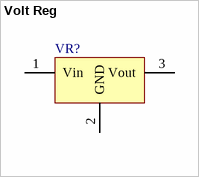
[diagram p0: symbol Volt Reg]
# Altium schematic symbol library MISC89340-2.SchLib: 1 symbol
Pins are listed as number, name and electrical type; pins without a type are passive.


## Volt Reg
designator VR?
Voltage Regulator
footprint 7805
pins: 1 Vin, 2 GND, 3 Vout